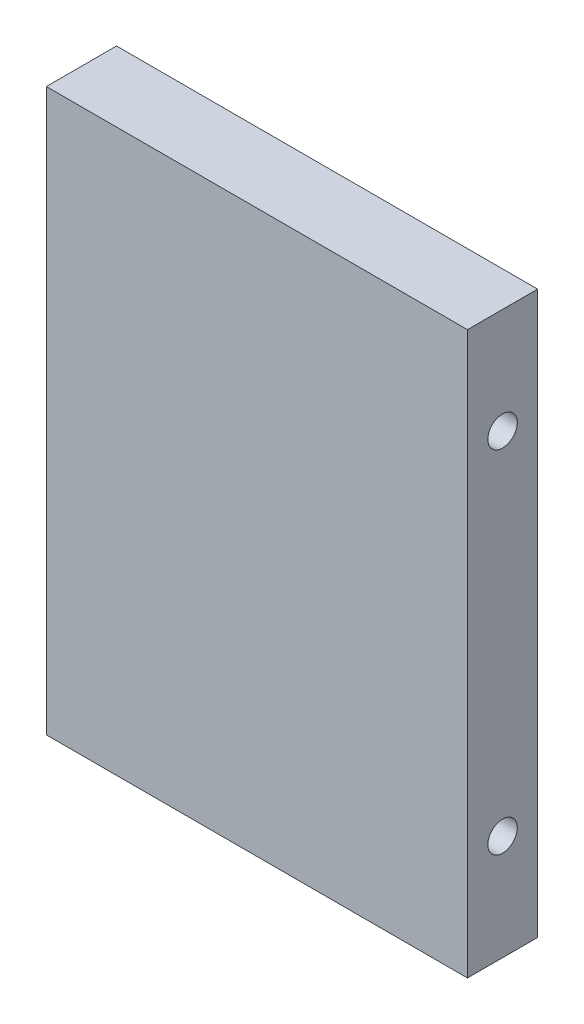
SolidWorks part; units mm, degrees
ref_plane "前视" through (0, 0, 0) normal (0, 0, 1) x (1, 0, 0)
ref_plane "上视" through (0, 0, 0) normal (0, 1, 0) x (1, 0, 0)
ref_plane "右视" through (0, 0, 0) normal (1, 0, 0) x (0, 0, -1)
sketch "草图1" plane through (0, 0, 0) normal (0, 0, 1) x (1, 0, 0)
  line L1 (-30, 40) -> (30, 40)
  line L2 (-30, 40) -> (-30, -40)
  line L3 (-30, -40) -> (30, -40)
  line L4 (30, 40) -> (30, -40)
  line L5 (-30, 40) -> (30, -40) construction
  line L6 (-30, -40) -> (30, 40) construction
  point P0 (0, 0)
  dimension "D1" = 60
  dimension "D2" = 80
extrude "凸台-拉伸1" add sketch "草图1" along normal blind 10
hole_wizard "M5 螺纹孔1" positions "草图3" profile "草图2" tap size "M5" standard "GB"
sketch "草图3" plane through (30, 0, 0) normal (1, 0, 0) x (0, 0, -1)
  line L0 (-5, -25) -> (-5, 25) construction
  line L3 (-5, 25) -> (-5, 40) construction
  line L4 (-10, 40) -> (0, 40) construction
  line L7 (-5, 0) -> (0, 0) construction
  line L8 (0, -40) -> (0, 40) construction
  point P0 (-5, -25)
  point P2 (-5, 25)
  dimension "D1" = 50
sketch "草图2" plane through (30, -25, 5) normal (0, 1, 0) x (0, 0, -1)
  line L0 (0, 0) -> (0, 15.2618)
  line L1 (0, 15.2618) -> (2.1, 14)
  line L2 (2.1, 14) -> (2.1, 0)
  line L5 (2.1, 0) -> (0, 0)
  line L10 (0, 15.2618) -> (-2.1, 14) construction
  line L11 (0, -6.35) -> (0, 107.95) construction
  dimension "螺纹孔钻头直径" = 4.2
  dimension "螺纹孔钻头深度" = 14
  dimension "导头角度" = 118
cosmetic thread "孔螺蚊线1" parameters "D1"=10, "D2"=5
cosmetic thread "孔螺蚊线2" parameters "D1"=10, "D2"=5
hole_wizard "M5 螺纹孔2" positions "草图5" profile "草图4" tap size "M5" standard "GB"
sketch "草图5" plane through (-30, 0, 0) normal (-1, 0, 0) x (0, 0, 1)
  point P0 (5, 25)
  point P3 (5, -25)
sketch "草图4" plane through (-30, 25, 5) normal (0, 1, 0) x (0, 0, 1)
  line L0 (0, 0) -> (0, 15.2618)
  line L1 (0, 15.2618) -> (2.1, 14)
  line L2 (2.1, 14) -> (2.1, 0)
  line L5 (2.1, 0) -> (0, 0)
  line L10 (0, 15.2618) -> (-2.1, 14) construction
  line L11 (0, -6.35) -> (0, 107.95) construction
  dimension "螺纹孔钻头直径" = 4.2
  dimension "螺纹孔钻头深度" = 14
  dimension "导头角度" = 118
cosmetic thread "孔螺蚊线3" parameters "D1"=10, "D2"=5
cosmetic thread "孔螺蚊线4" parameters "D1"=10, "D2"=5
